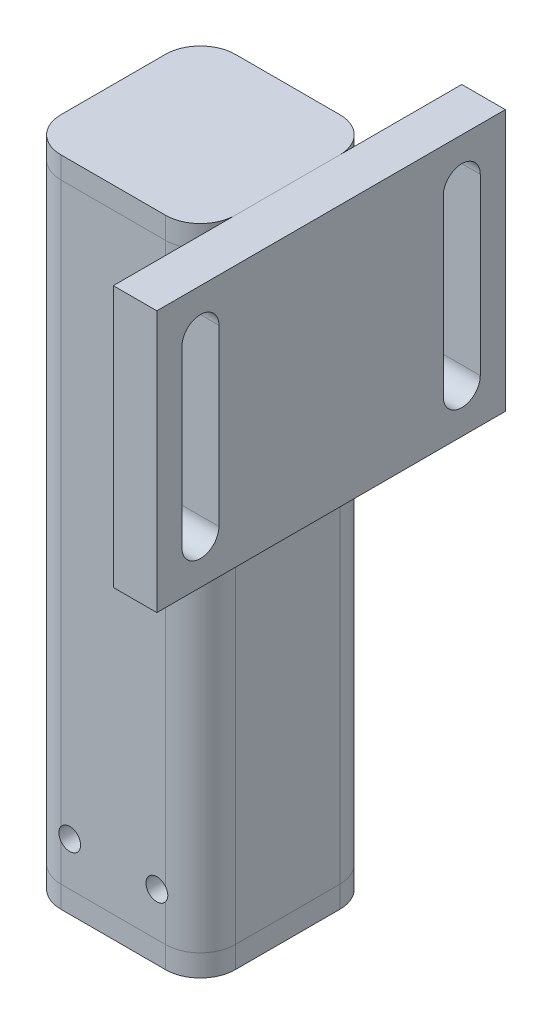
from build123d import *

# Parameters (mm, degrees)
F_40_X_40_X_4_0_1_DEPTH     = 150
SKETCH_3_W                  = 80
SKETCH_3_H                  = 60
EXTRUDE_1_DEPTH             = 10
CUT_EXTRUDE_2_DEPTH         = 164.095064303
SKETCH_14_W                 = 2.5
SKETCH_14_H                 = 60
HOLE_WIZARD_M6_1_AT_2_COUNT = 2
HOLE_WIZARD_M6_1_AT_2_PITCH = 20
END_CAP_1_THICKNESS         = 5
HOLE_WIZARD_M6_2_AT_2_COUNT = 2
HOLE_WIZARD_M6_2_AT_2_PITCH = 20
END_CAP_2_THICKNESS         = 5


with BuildPart() as part:
    # Sketch1 → 方管 40 X 40 X 4.0(1) (new body)
    with BuildSketch(Plane.ZX):
        with BuildLine():
            Line((-12, -20), (12, -20))
            ThreePointArc((12, -20), (17.656854249, -17.656854249), (20, -12))
            Line((20, -12), (20, 12))
            ThreePointArc((20, 12), (17.656854249, 17.656854249), (12, 20))
            Line((12, 20), (-12, 20))
            ThreePointArc((-12, 20), (-17.656854249, 17.656854249), (-20, 12))
            Line((-20, 12), (-20, -12))
            ThreePointArc((-20, -12), (-17.656854249, -17.656854249), (-12, -20))
        make_face()
        with BuildLine():
            Line((-12, -16), (12, -16))
            ThreePointArc((12, -16), (14.828427125, -14.828427125), (16, -12))
            Line((16, -12), (16, 12))
            ThreePointArc((16, 12), (14.828427125, 14.828427125), (12, 16))
            Line((12, 16), (-12, 16))
            ThreePointArc((-12, 16), (-14.828427125, 14.828427125), (-16, 12))
            Line((-16, 12), (-16, -12))
            ThreePointArc((-16, -12), (-14.828427125, -14.828427125), (-12, -16))
        make_face(mode=Mode.SUBTRACT)
    extrude(amount=F_40_X_40_X_4_0_1_DEPTH)

    # 草图14 → M6 螺纹孔1 (revolve, cut)
    with BuildSketch(Plane(origin=(-10, 15, 20), x_dir=(0, -1, 0), z_dir=(1, 0, 0))):
        with Locations((1.25, 30)):
            Rectangle(SKETCH_14_W, SKETCH_14_H)
    hole_wizard_m6_1 = revolve(axis=Axis((-10, 15, 26.35), (0, 0, -1)), mode=Mode.SUBTRACT)

    # M6 螺纹孔1 at 2: M6 螺纹孔1 ×2
    with Locations(*[(i * HOLE_WIZARD_M6_1_AT_2_PITCH, 0, 0) for i in range(1, HOLE_WIZARD_M6_1_AT_2_COUNT)]):
        add(hole_wizard_m6_1, mode=Mode.SUBTRACT)


with BuildPart() as body_2:
    # 草图3 → 凸台-拉伸1 (new body)
    with BuildSketch(Plane(origin=(20, 0, 0), x_dir=(0, 0, -1), z_dir=(1, 0, 0))):
        with Locations((0, 120)):
            Rectangle(SKETCH_3_W, SKETCH_3_H)
    extrude(amount=EXTRUDE_1_DEPTH)

    # 草图12 → 切除-拉伸2 (cut, through all)
    with BuildSketch(Plane(origin=(30, 0, 0), x_dir=(0, 0, -1), z_dir=(1, 0, 0))):
        with BuildLine():
            Line((-25.75, 140), (-25.75, 100))
            ThreePointArc((-25.75, 100), (-30, 95.75), (-34.25, 100))
            Line((-34.25, 100), (-34.25, 140))
            ThreePointArc((-34.25, 140), (-30, 144.25), (-25.75, 140))
        make_face()
        with BuildLine():
            Line((34.25, 140), (34.25, 100))
            ThreePointArc((34.25, 100), (30, 95.75), (25.75, 100))
            Line((25.75, 100), (25.75, 140))
            ThreePointArc((25.75, 140), (30, 144.25), (34.25, 140))
        make_face()
    extrude(amount=-CUT_EXTRUDE_2_DEPTH, mode=Mode.SUBTRACT)


with BuildPart() as body_3:
    # End Cap 1: an end cap: a plate 5.0 thick on the member's open end, its outline the end's outer outline
    end_cap_1_end = part.part.faces().sort_by_distance((-16, 0, -16))[0]
    add(extrude(Face(end_cap_1_end.outer_wire()), amount=END_CAP_1_THICKNESS, dir=(0, 1, 0)))

    # 草图17 → M6 螺纹孔2 (revolve, cut)
    with BuildSketch(Plane(origin=(-10, 0, 0), x_dir=(0, 0, -1), z_dir=(1, 0, 0))):
        Polygon((0, 0), (0, 16.502151548), (2.5, 15), (2.5, 0), align=None)
    hole_wizard_m6_2 = revolve(axis=Axis((-10, -6.35, 0), (0, 1, 0)), mode=Mode.SUBTRACT)

    # M6 螺纹孔2 at 2: M6 螺纹孔2 ×2
    with Locations(*[(i * HOLE_WIZARD_M6_2_AT_2_PITCH, 0, 0) for i in range(1, HOLE_WIZARD_M6_2_AT_2_COUNT)]):
        add(hole_wizard_m6_2, mode=Mode.SUBTRACT)


with BuildPart() as part_1:
    add(part.part)

    # End Cap 1 3
    split(bisect_by=Plane(origin=(0, 5, 0), x_dir=(-1, 0, 0), z_dir=(0, 1, 0)), keep=Keep.TOP)


with BuildPart() as body_4:
    # End Cap 2: an end cap: a plate 5.0 thick on the member's open end, its outline the end's outer outline
    end_cap_2_end = part_1.part.faces().sort_by_distance((-16, 150, -16))[0]
    add(extrude(Face(end_cap_2_end.outer_wire()), amount=END_CAP_2_THICKNESS, dir=(0, -1, 0)))


with BuildPart() as part_2:
    add(part_1.part)

    # End Cap 2 3
    split(bisect_by=Plane.XZ.offset(-145), keep=Keep.TOP)


solid = Compound([body_2.part, body_3.part, body_4.part, part_2.part])
